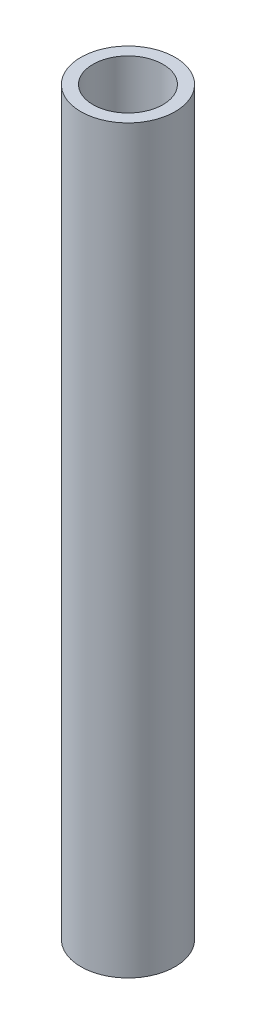
from build123d import *

# Parameters (mm, degrees)
SKETCH_1_R      = 17.5
EXTRUDE_1_DEPTH = 275
SHELL_1_T       = -4.5


with BuildPart() as part:
    # 草图1 → 凸台-拉伸1 (new body)
    with BuildSketch(Plane(origin=(0, 0, 0), x_dir=(1, 0, 0), z_dir=(0, 1, 0))):
        with Locations(Location((0, 0, 0), (0, 0, 270))):
            Circle(SKETCH_1_R)
    extrude(amount=EXTRUDE_1_DEPTH)

    # 抽壳1
    shell_1_openings = [part.faces().sort_by_distance(p)[0] for p in [
        (0, 275, 0),
        (0, 0, 0),
    ]]
    offset(amount=SHELL_1_T, openings=shell_1_openings, kind=Kind.INTERSECTION)


solid = part.part
